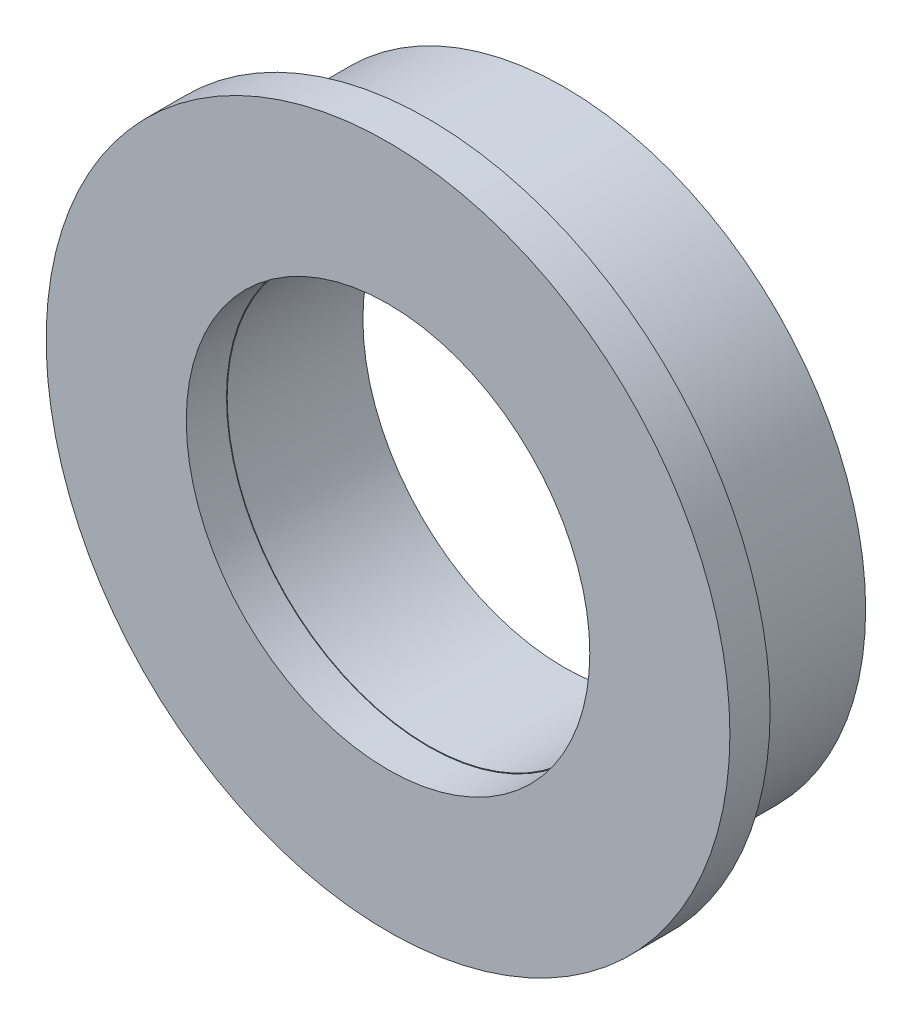
from build123d import *

# Parameters (mm, degrees)
SKETCH_1_R      = 6
SKETCH_1_R_2    = 4
EXTRUDE_1_DEPTH = 2.7
SKETCH_2_R      = 6.8
SKETCH_2_R_2    = 4.013379479
EXTRUDE_2_DEPTH = 0.8


with BuildPart() as part:
    # 草图1 → 凸台-拉伸1 (new body)
    with BuildSketch(Plane.XY):
        with Locations(Location((0, 0, 0), (0, 0, 180))):
            Circle(SKETCH_1_R)
        with Locations(Location((0, 0, 0), (0, 0, 180))):
            Circle(SKETCH_1_R_2, mode=Mode.SUBTRACT)
    extrude(amount=EXTRUDE_1_DEPTH)

    # 草图2 → 凸台-拉伸2 (add)
    with BuildSketch(Plane.XY.offset(2.7)):
        Circle(SKETCH_2_R)
        Circle(SKETCH_2_R_2, mode=Mode.SUBTRACT)
    extrude(amount=EXTRUDE_2_DEPTH)


solid = part.part
